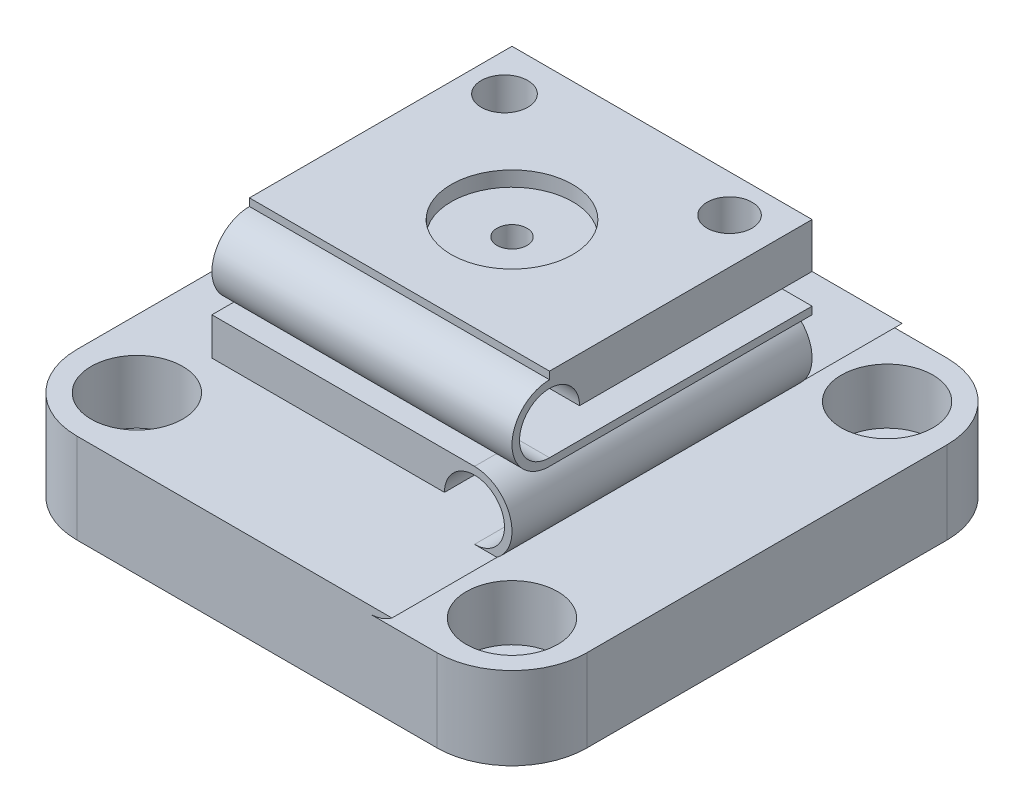
from build123d import *

# Parameters (mm, degrees)
SKETCH1_W           = 34
SKETCH1_H           = 34
BOSS_EXTRUDE1_DEPTH = 6
SKETCH2_R           = 1.6
CUT_EXTRUDE1_DEPTH  = 6
SKETCH3_R           = 3.05
CUT_EXTRUDE2_DEPTH  = 4.2
SKETCH4_W           = 20
SKETCH4_H           = 20
BOSS_EXTRUDE2_DEPTH = 10
CUT_EXTRUDE4_DEPTH  = 42.243181255
CUT_EXTRUDE5_DEPTH  = 36.693136595
SKETCH7_R           = 1.5
CUT_EXTRUDE6_DEPTH  = 4
FILLET1_R           = 5
SKETCH8_R           = 1
CUT_EXTRUDE7_DEPTH  = 4
SKETCH9_R           = 4.05
CUT_EXTRUDE8_DEPTH  = 1
SKETCH10_R          = 1.55
CUT_EXTRUDE9_DEPTH  = 9


with BuildPart() as part:
    # Sketch1 → Boss-Extrude1 (new body)
    with BuildSketch(Plane(origin=(0, 0, 0), x_dir=(1, 0, 0), z_dir=(0, 1, 0))):
        Rectangle(SKETCH1_W, SKETCH1_H)
    extrude(amount=BOSS_EXTRUDE1_DEPTH)

    # Sketch2 → Cut-Extrude1 (cut)
    with BuildSketch(Plane(origin=(0, 6, 0), x_dir=(1, 0, 0), z_dir=(0, 1, 0))):
        with Locations(Location((-12.5, 12.5, 0), (0, 0, 270))):
            Circle(SKETCH2_R)
        with Locations(Location((12.5, 12.5, 0), (0, 0, 270))):
            Circle(SKETCH2_R)
        with Locations(Location((12.5, -12.5, 0), (0, 0, 270))):
            Circle(SKETCH2_R)
        with Locations(Location((-12.5, -12.5, 0), (0, 0, 270))):
            Circle(SKETCH2_R)
    extrude(amount=-CUT_EXTRUDE1_DEPTH, mode=Mode.SUBTRACT)

    # Sketch3 → Cut-Extrude2 (cut)
    with BuildSketch(Plane(origin=(0, 6, 0), x_dir=(1, 0, 0), z_dir=(0, 1, 0))):
        with Locations(Location((-12.5, 12.5, 0), (0, 0, 270))):
            Circle(SKETCH3_R)
        with Locations(Location((12.5, 12.5, 0), (0, 0, 270))):
            Circle(SKETCH3_R)
        with Locations(Location((12.5, -12.5, 0), (0, 0, 270))):
            Circle(SKETCH3_R)
        with Locations(Location((-12.5, -12.5, 0), (0, 0, 270))):
            Circle(SKETCH3_R)
    extrude(amount=-CUT_EXTRUDE2_DEPTH, mode=Mode.SUBTRACT)

    # Sketch4 → Boss-Extrude2 (add)
    with BuildSketch(Plane(origin=(0, 6, 0), x_dir=(1, 0, 0), z_dir=(0, 1, 0))):
        Rectangle(SKETCH4_W, SKETCH4_H)
    extrude(amount=BOSS_EXTRUDE2_DEPTH)

    # Sketch5 → Cut-Extrude4 (cut, through all)
    with BuildSketch(Plane.XY.offset(17)):
        with BuildLine():
            Line((-10, 6), (7.5, 6))
            ThreePointArc((7.5, 6), (8.914213562, 9.414213562), (5.5, 8))
            Line((5.5, 8), (-10, 8))
            Line((-10, 8), (-10, 6))
        make_face()
        with BuildLine():
            Line((10, 10.5), (7.5, 10.5))
            ThreePointArc((7.5, 10.5), (9.267766953, 9.767766953), (10, 8))
            Line((10, 8), (10, 10.5))
        make_face()
        with BuildLine():
            Line((10, 6), (10, 8))
            ThreePointArc((10, 8), (9.736067977, 6.881966011), (9, 6))
            Line((9, 6), (10, 6))
        make_face()
        with BuildLine():
            Line((17, 6), (10, 6))
            Line((10, 6), (9, 6))
            ThreePointArc((9, 6), (8.290569415, 5.628291755), (7.5, 5.5))
            Line((7.5, 5.5), (17, 5.5))
            Line((17, 5.5), (17, 6))
        make_face()
    extrude(amount=-CUT_EXTRUDE4_DEPTH, mode=Mode.SUBTRACT)

    # Sketch6 → Cut-Extrude5 (cut, through all)
    with BuildSketch(Plane.ZY.offset(10)):
        with BuildLine():
            ThreePointArc((10, 13), (9.267766953, 11.232233047), (7.5, 10.5))
            Line((7.5, 10.5), (10, 10.5))
            Line((10, 10.5), (10, 13))
        make_face()
        with BuildLine():
            ThreePointArc((7.5, 15.5), (9.267766953, 14.767766953), (10, 13))
            Line((10, 13), (10, 16))
            Line((10, 16), (7.5, 16))
            Line((7.5, 16), (7.5, 15.5))
        make_face()
        with BuildLine():
            Line((-10, 13), (-10, 11))
            Line((-10, 11), (7.5, 11))
            ThreePointArc((7.5, 11), (8.914213562, 14.414213562), (5.5, 13))
            Line((5.5, 13), (-10, 13))
        make_face()
    extrude(amount=-CUT_EXTRUDE5_DEPTH, mode=Mode.SUBTRACT)

    # Sketch7 → Cut-Extrude6 (cut)
    with BuildSketch(Plane(origin=(0, 16, 0), x_dir=(1, 0, 0), z_dir=(0, 1, 0))):
        with Locations(Location((7, 7.5, 0), (0, 0, 270))):
            Circle(SKETCH7_R)
    extrude(amount=-CUT_EXTRUDE6_DEPTH, mode=Mode.SUBTRACT)

    # Fillet1
    fillet1_edges = [part.edges().sort_by_distance(p)[0] for p in [
        (17, 2.75, 17),
        (17, 2.75, -17),
        (-17, 3, 17),
        (-17, 3, -17),
    ]]
    fillet(fillet1_edges, radius=FILLET1_R)

    # Sketch8 → Cut-Extrude7 (cut)
    with BuildSketch(Plane(origin=(0, 16, 0), x_dir=(1, 0, 0), z_dir=(0, 1, 0))):
        with Locations(Location((0, 0, 0), (0, 0, 270))):
            Circle(SKETCH8_R)
    extrude(amount=-CUT_EXTRUDE7_DEPTH, mode=Mode.SUBTRACT)

    # Sketch9 → Cut-Extrude8 (cut)
    with BuildSketch(Plane(origin=(0, 16, 0), x_dir=(1, 0, 0), z_dir=(0, 1, 0))):
        with Locations(Location((0, 0, 0), (0, 0, 270))):
            Circle(SKETCH9_R)
    extrude(amount=-CUT_EXTRUDE8_DEPTH, mode=Mode.SUBTRACT)

    # Sketch10 → Cut-Extrude9 (cut)
    with BuildSketch(Plane(origin=(0, 16, 0), x_dir=(1, 0, 0), z_dir=(0, 1, 0))):
        with Locations(Location((-7.5, 7, 0), (0, 0, 270))):
            Circle(SKETCH10_R)
    extrude(amount=-CUT_EXTRUDE9_DEPTH, mode=Mode.SUBTRACT)


solid = part.part
